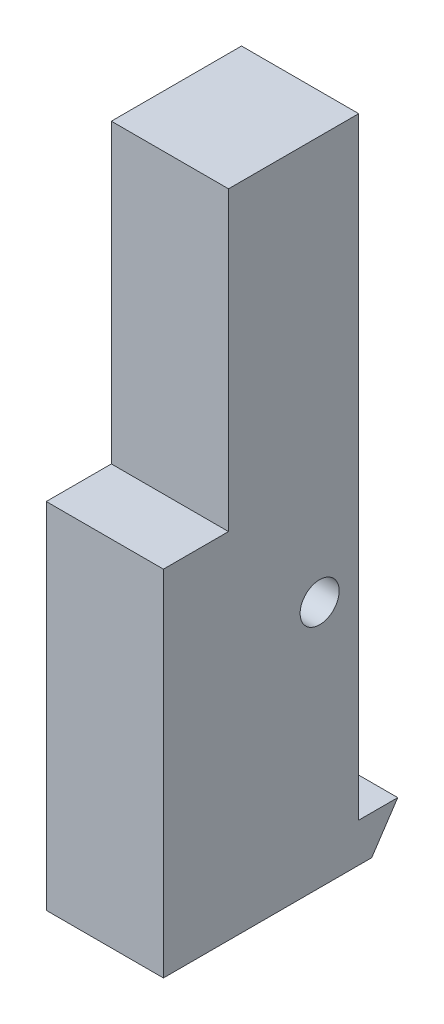
SolidWorks part; units mm, degrees
material "不锈钢花纹钣金"
ref_plane "Front Plane" through (0, 0, 0) normal (0, 0, 1) x (1, 0, 0)
ref_plane "Top Plane" through (0, 0, 0) normal (0, 1, 0) x (1, 0, 0)
ref_plane "Right Plane" through (0, 0, 0) normal (1, 0, 0) x (0, 0, -1)
sketch "Sketch43" plane through (0, 0, 0) normal (0, 0, 1) x (1, 0, 0)
  line L1 (-2.25, 12.5) -> (2.25, 12.5)
  line L2 (-2.25, 12.5) -> (-2.25, -12.5)
  line L3 (-2.25, -12.5) -> (2.25, -12.5)
  line L4 (2.25, 12.5) -> (2.25, -12.5)
  line L5 (-2.25, 12.5) -> (2.25, -12.5) construction
  line L6 (-2.25, -12.5) -> (2.25, 12.5) construction
  point P0 (0, 0)
  dimension "D1" = 4.5
  dimension "D2" = 25
extrude "Boss-Extrude1" add sketch "Sketch43" along normal blind 7.5
sketch "Sketch44" plane through (2.25, 0, 0) normal (1, 0, 0) x (0, 0, -1)
  line L0 (0, -12.5) -> (0.5, -12.5)
  line L1 (0.5, -12.5) -> (1.5, -11)
  line L2 (1.5, -11) -> (0, -11)
  line L3 (-10, -11) -> (0, -11) construction
  line L4 (0, 14) -> (0, -11) construction
  line L5 (0, -12.5) -> (0, -11)
  dimension "D1" = 1.5
  dimension "D2" = 0.5
extrude "Boss-Extrude2" add sketch "Sketch44" against normal up to surface (4.5 mm away) up to face at (-2.25, 0, 3.75)
sketch "Sketch45" plane through (2.25, 0, 0) normal (1, 0, 0) x (0, 0, -1)
  circle A0 centre (-1.5, -3) radius 0.75 construction
  circle A1 centre (-1.5, -3) radius 0.75
extrude "Cut-Extrude1" cut sketch "Sketch45" against normal through all
sketch "Sketch46" plane through (-2.25, 0, 0) normal (-1, 0, 0) x (0, 0, 1)
  line L1 (7.5, 12.5) -> (5, 12.5)
  line L2 (7.5, 12.5) -> (7.5, 1.0994)
  line L3 (7.5, 1.0994) -> (5, 1.0994)
  line L4 (5, 12.5) -> (5, 1.0994)
  dimension "D1" = 2.5
extrude "Cut-Extrude2" cut sketch "Sketch46" against normal through all
